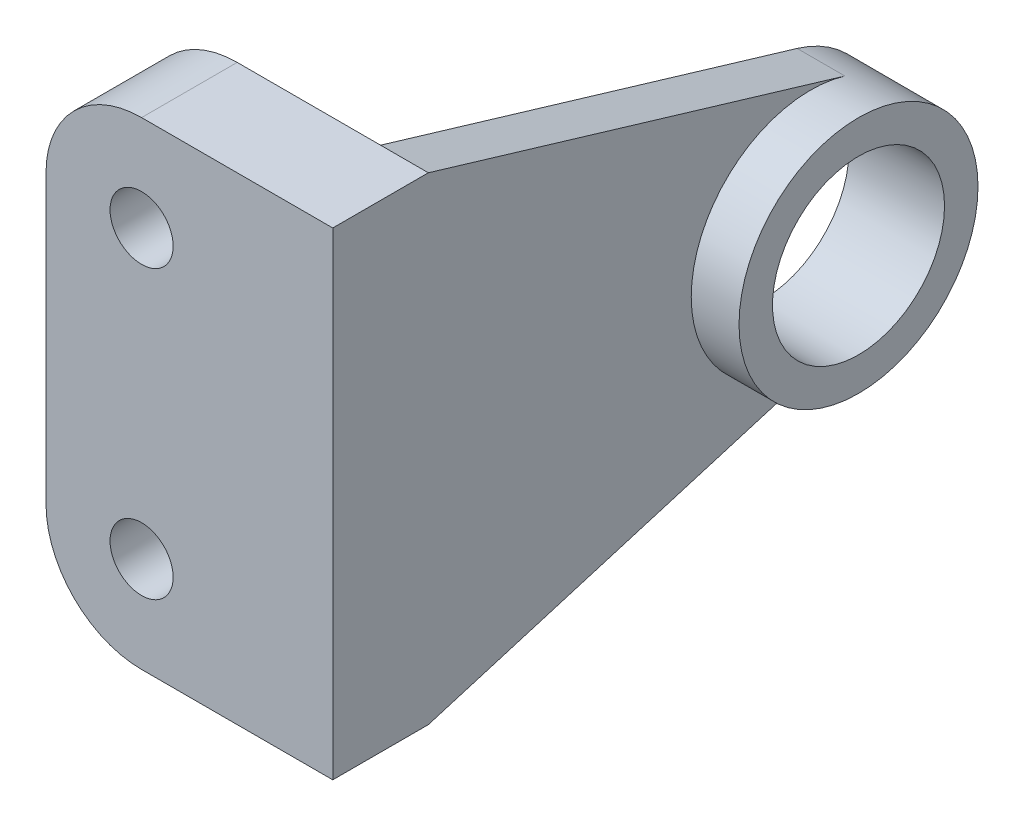
SolidWorks part; units mm, degrees
other "Annotation1"
sketch "草图6" plane through (-15, -25, -52.5) normal (-0.0479, -0.5543, -0.831) x (-0.8441, 0.4672, -0.263)
ref_plane "Front Plane" through (0, 0, 0) normal (0, 0, 1) x (1, 0, 0)
ref_plane "Top Plane" through (0, 0, 0) normal (0, 1, 0) x (1, 0, 0)
ref_plane "Right Plane" through (0, 0, 0) normal (1, 0, 0) x (0, 0, -1)
sketch "Sketch1" plane through (0, 0, 0) normal (0, 0, 1) x (1, 0, 0)
  line L1 (-15, -25) -> (15, -25)
  line L2 (-15, -25) -> (-15, 25)
  line L3 (-15, 25) -> (15, 25)
  line L4 (15, -25) -> (15, 25)
  line L5 (-15, -25) -> (15, 25) construction
  line L6 (-15, 25) -> (15, -25) construction
  point P0 (0, 0)
  dimension "D1" = 30
  dimension "D2" = 50
extrude "Boss-Extrude1" add sketch "Sketch1" along normal blind 10
sketch "Sketch2" plane through (15, -15, 0) normal (-1, 0, 0) x (0, 1, 0)
  line L6 (3.0234, 43.5791) -> (-10, 0)
  line L7 (26.9766, 43.5791) -> (40, 0)
  line L8 (-10, 0) -> (40, 0)
  line L9 (40, -10) -> (-10, -10) construction
  circle A0 centre (15, 40) radius 9
  arc A1 (26.9766, 43.5791) -> (3.0234, 43.5791) centre (15, 40) ccw
  dimension "D1" = 18
  dimension "D2" = 25
  dimension "D3" = 50
extrude "Boss-Extrude3" add sketch "Sketch2" along normal blind 5
sketch "Sketch3" plane through (15, 0, 0) normal (1, 0, 0) x (0, 0, -1)
  circle A0 centre (40, 0) radius 9
  circle A1 centre (40, 0) radius 12.5
  dimension "D1" = 25
  dimension "D2" = 18
extrude "Boss-Extrude4" add sketch "Sketch3" along normal blind 5
fillet "Fillet1" radius 10 2 edges at (-15, 25, 5) (-15, -25, 5)
hole_wizard "CBORE for M6 Hexagon socket head cap screws1" positions "3DSketch1" profile "Sketch4" counterbore size "M6" standard "GB"
sketch3d "3DSketch1"
  line L0 (-5, -15, 10) -> (-5, -15, 0) construction
  line L1 (-5, 15, 10) -> (-5, 15, 0) construction
  point P0 (-5, -15, 0)
  point P4 (-5, 15, 0)
sketch "Sketch4" plane through (-5, -15, 0) normal (1, 0, 0) x (0, 1, 0)
  line L0 (0, 0) -> (0, 5)
  line L1 (0, 5) -> (3.3, 3.0172)
  line L2 (3.3, 3.0172) -> (3.3, 5)
  line L3 (3.3, 5) -> (5.5, 5)
  line L4 (5.5, 5) -> (5.5, 0)
  line L5 (5.5, 0) -> (0, 0)
  line L10 (0, 5) -> (-3.3, 3.0172) construction
  line L11 (0, -6.35) -> (0, 107.95) construction
  dimension "孔直径" = 6.6
  dimension "孔深度" = 5
  dimension "柱形沉头孔直径" = 11
  dimension "柱形沉头孔深度" = 5
  dimension "导头角度" = 118
sketch "Sketch8" plane through (0, 0, 5) normal (0, 0, -1) x (-1, 0, 0)
  circle A0 centre (5, -15) radius 3.3 construction
  circle A1 centre (5, 15) radius 3.3 construction
  circle A2 centre (5, -15) radius 3.3
  circle A3 centre (5, 15) radius 3.3
extrude "Cut-Extrude1" cut sketch "Sketch8" against normal blind 19 and the other way blind 27
